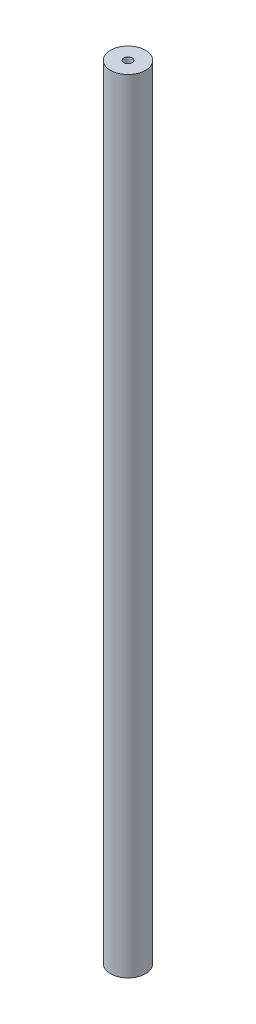
SolidWorks part; units mm, degrees
material "ABS"
ref_plane "Front Plane" through (0, 0, 0) normal (0, 0, 1) x (1, 0, 0)
ref_plane "Top Plane" through (0, 0, 0) normal (0, 1, 0) x (1, 0, 0)
ref_plane "Right Plane" through (0, 0, 0) normal (1, 0, 0) x (0, 0, -1)
sketch "Sketch1" plane through (0, 0, 0) normal (0, 0, 1) x (1, 0, 0)
  line L0 (0, -3.5684) -> (0, 52.4487) construction
  line L1 (-1.05, 0) -> (-0.25, 0)
  line L2 (-1.05, 0) -> (-1.05, 47)
  line L3 (-1.05, 47) -> (-0.25, 47)
  line L4 (-0.25, 0) -> (-0.25, 47)
  dimension "D1" = 2.1
  dimension "D2" = 0.5
  dimension "D3" = 47
revolve "Revolve1" add sketch "Sketch1" angle 360 about L0
